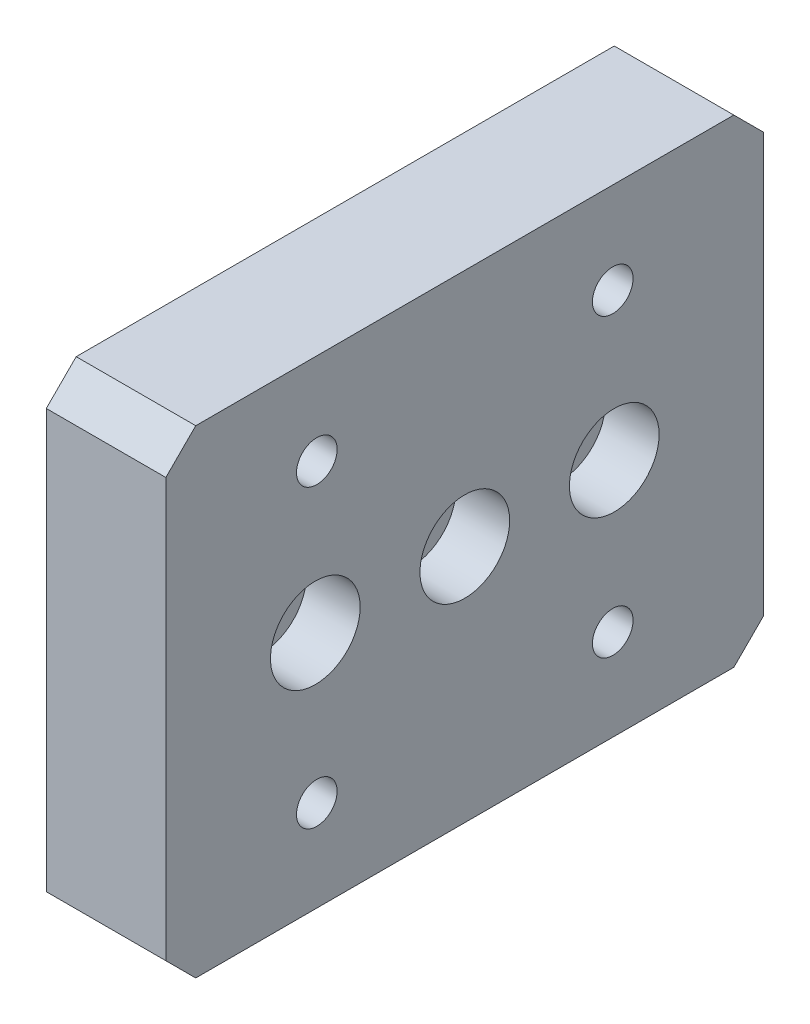
SolidWorks part; units mm, degrees
ref_plane "前视基准面" through (0, 0, 0) normal (0, 0, 1) x (1, 0, 0)
ref_plane "上视基准面" through (0, 0, 0) normal (0, 1, 0) x (1, 0, 0)
ref_plane "右视基准面" through (0, 0, 0) normal (1, 0, 0) x (0, 0, -1)
sketch "草图1" plane through (0, 0, 0) normal (1, 0, 0) x (0, 0, -1)
  line L1 (-50, 40) -> (50, 40)
  line L2 (-50, 40) -> (-50, -40)
  line L3 (-50, -40) -> (50, -40)
  line L4 (50, 40) -> (50, -40)
  line L5 (-50, 40) -> (50, -40) construction
  line L6 (-50, -40) -> (50, 40) construction
  point P0 (0, 0)
  dimension "D1" = 100
  dimension "D2" = 80
extrude "凸台-拉伸1" add sketch "草图1" along normal blind 20
hole_wizard "M8 螺纹孔1" positions "草图2" profile "草图3" tap size "M8" standard "GB" end condition through all
sketch "草图2" plane through (20, 0, 0) normal (1, 0, 0) x (0, 0, -1)
  line L0 (-24.7487, 24.7487) -> (0, 0) construction
  line L1 (0, 0) -> (0, 56.449) construction
  point P0 (-24.7487, 24.7487)
  point P13 (24.7487, 24.7487)
  point P14 (24.7487, -24.7487)
  point P15 (-24.7487, -24.7487)
  dimension "D1" = 45
  dimension "D2" = 35
  dimension "D3" = 4
sketch "草图3" plane through (20, 24.7487, 24.7487) normal (0, 1, 0) x (0, 0, -1)
  line L0 (0, 0) -> (0, 20)
  line L1 (0, 20) -> (3.4, 20)
  line L2 (3.4, 20) -> (3.4, 0)
  line L5 (3.4, 0) -> (0, 0)
  line L11 (0, -6.35) -> (0, 107.95) construction
  dimension "通孔螺纹孔钻头直径" = 6.8
  dimension "通孔螺纹孔钻头深度" = 20
cosmetic thread "孔螺蚊线1" parameters "D2"=8
cosmetic thread "孔螺蚊线2" parameters "D2"=8
cosmetic thread "孔螺蚊线3" parameters "D2"=8
cosmetic thread "孔螺蚊线4" parameters "D2"=8
hole_wizard "打孔尺寸(%根据)内六角圆柱头螺钉的类型1" positions "草图4" profile "草图5" counterbore size "M8" standard "GB" end condition through all
sketch "草图4" plane through (20, 0, 0) normal (1, 0, 0) x (0, 0, -1)
  line L0 (0, -40) -> (0, 44.8333) construction
  line L1 (-50, -40) -> (50, -40) construction
  point P0 (-25, 0)
  point P2 (0, 0)
  point P5 (25, 0)
  dimension "D1" = 50
sketch "草图5" plane through (20, 0, 25) normal (0, 1, 0) x (0, 0, -1)
  line L0 (0, 0) -> (0, 20)
  line L1 (0, 20) -> (4.5, 20)
  line L3 (4.5, 20) -> (4.5, 9)
  line L4 (4.5, 9) -> (7.5, 9)
  line L5 (7.5, 9) -> (7.5, 0)
  line L7 (7.5, 0) -> (0, 0)
  line L11 (0, -6.35) -> (0, 107.95) construction
  dimension "通孔孔直径" = 9
  dimension "通孔孔深度" = 20
  dimension "柱形沉头孔直径" = 15
  dimension "柱形沉头孔深度" = 9
chamfer "倒角1" distance 5 angle 45 4 edges at (10, 40, -50) (10, -40, -50) (10, 40, 50) (10, -40, 50)
